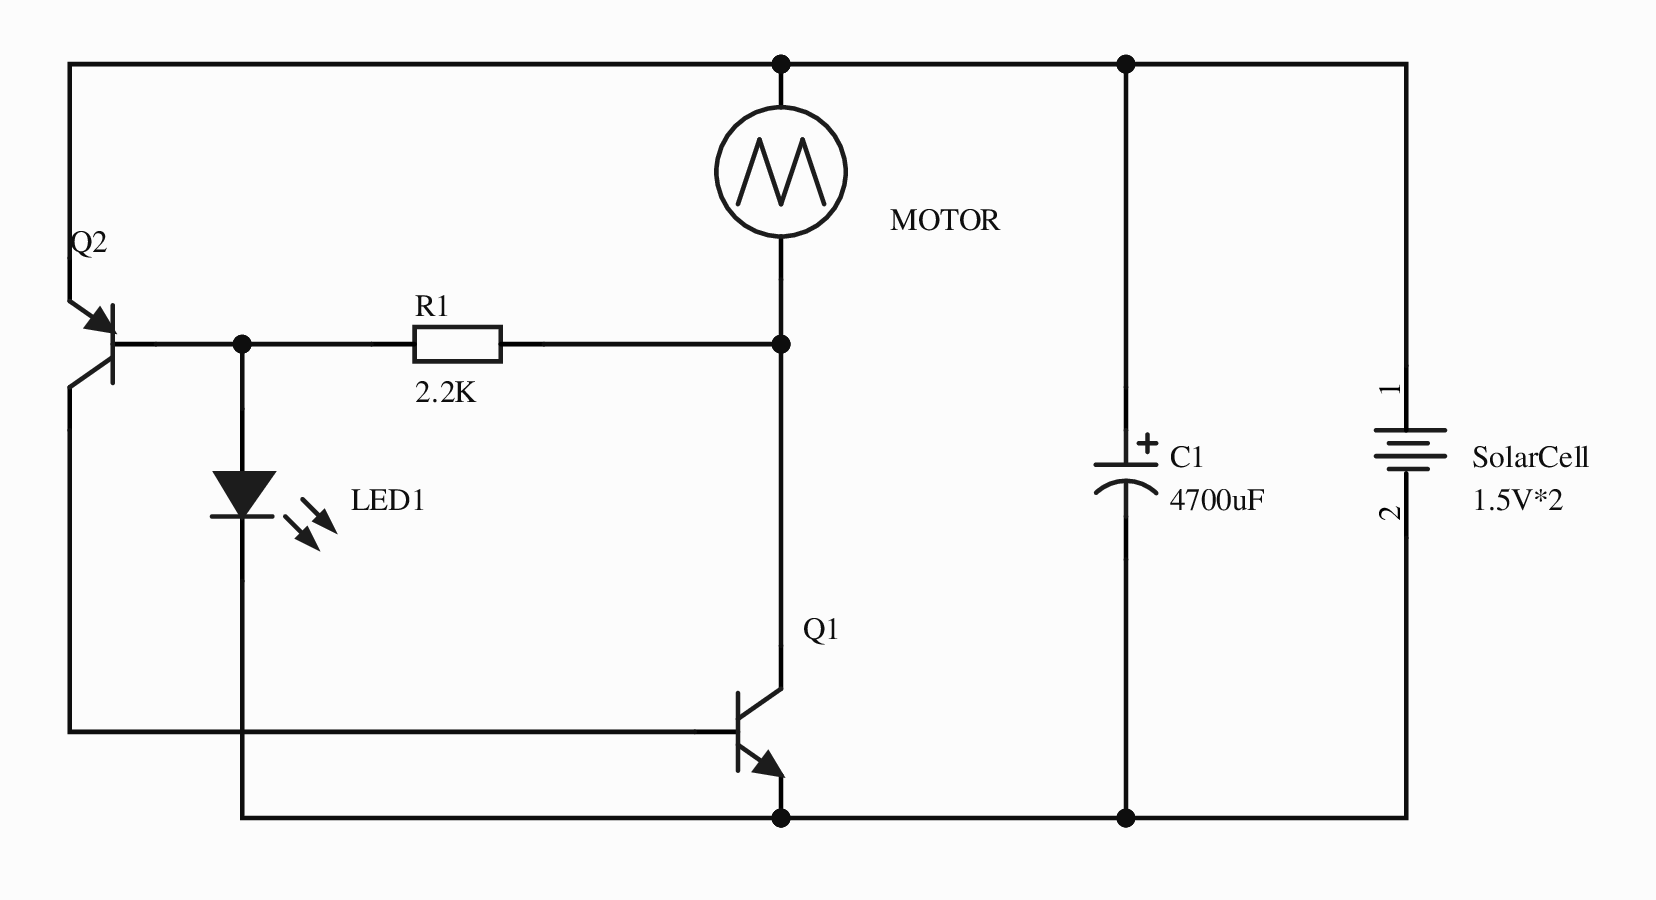
[diagram p0: MISC49939-3.schdoc]
# Altium project MISC49939-2.PrjPcb
1 sheet, 7 parts. Net scope: global (net labels, ports and power ports of the same name join across sheets).
Board file: MISC49939.pcbdoc

## Sheet MISC49939-3.schdoc
size 297 x 209 mm; Version: V1.0; @Project Name: MISC49939; @Update Date: 2026-10-05; @Create Date: 2026-10-05; @Board Name: MISC49939; @Create Time: 20:24:00; @Page Count: 1; @Page No: 1; @Schematic Name: MISC49939; @Update Time: 20:24:00; Size: A4

### Parts
C1  4700uF  [CAP-TH_BD5.0-P2.00-D0.8-FD-10UF50VC110GL]
LED1  (no value)  [LED_0603]
MOTOR  MOTOR_3  [VIBRATING-MOTOR-SMD_3P_C9900012555]  (value not drawn)
Q1  (no value)  [S8050_SOT-23]
Q2  (no value)  [S8550P_SOT]
R1  2.2K  [R0603]
SolarCell  1.5V*2  [BAT-TH_CR2032-2-1]

### Nets
NetC1_1: C1.1 MOTOR.1 Q2.2(E) SolarCell.1
NetC1_2: C1.2 LED1.1(C) Q1.2 SolarCell.2
NetLED1_2: LED1.2(A) Q2.1(B) R1.1
NetMOTOR_2: MOTOR.2 Q1.3 R1.2
NetQ1_1: Q1.1 Q2.3(C)

### Library data of the parts
C1 = 10UF50VC110GL: Capacitance:10uF;Tolerance:±20%;Rated voltage:50V;Ripple current:120mA@100KHz;Equivalent series resistance(ESR):1.6Ω;; Manufacturer: Econd(米朗电子); AddInBom: yes; ModelId: b35ab6b0460c4c43a629d91cfc2b58780819f05c4eef4c71ace90d822a990e87; ModelTransform: 196.85,196.85,0,0,0,0,0,0,-196.85; Tolerance: ±20%; Voltage Rating: 50V; Equivalent Series Resistance(ESR): 1.6Ω; Pin Spacing: 2mm; Lifetime: 5000hrs@105℃; Symbol: 10UF50VC110GL; Device: 10UF50VC110GL; Value: 4700uF; FootprintName: CAP-TH_BD5.0-P2.00-D0.8-FD-10UF50VC110GL; LCSC Part Name: 10uF ±20% 50V; ManufacturerPart: 10UF50VC110GL; Supplier Footprint: 插件,D5xL11mm; JLCPCB Part Class: Extended Part; Datasheet: example.com/datasheet/10UF50VC110GL/49031974.html; Supplier: LCSC; ConvertToPcb: yes; ModelName: CAP-TH_BD5.0-P2.00-D0.8-FD-10UF50VC110GL; Ripple Current: 120mA@100KHz; Diameter: 5mm; Height - Seated (Max): 11mm; Operating Temperature: -40℃~+105℃
LED1 = LED_0603-B: Symbol: LED_B; Convert to PCB: yes; 3D Model: eb8d964598f24248affda46f619856c50819f05c4eef4c71ace90d822a990e87; 3D Model Transform: 63.1,31.6,23.7,0,0,0,0,0,0; ModelName: LED-0603_B; Device: LED_0603-B; Add into BOM: yes; Supplier Footprint: 0603; FootprintName: LED_0603
MOTOR = MOTOR_3: AddInBom: yes; Symbol: MOTOR_3; Device: MOTOR_3; FootprintName: VIBRATING-MOTOR-SMD_3P_C9900012555; LCSC Part Name: MOTOR_3; SupplierPart: C9900022375; ManufacturerPart: MOTOR_3; Supplier Footprint: SHOCK_0408; JLCPCB Part Class: Extended Part; Supplier: LCSC; ConvertToPcb: yes
Q1 = S8050_SOT_NPN: Symbol: NPN; ConvertToPcb: yes; ModelId: c62791f0466c4ae2a892c056b845b0ca0819f05c4eef4c71ace90d822a990e87; ModelName: SOT-23-3P_L2.9-W1.3-H1.0-LS2.4-P0.95; ModelTransform: 98.6,114.12,41.29,180,0,0,0,0,-3; Device: S8050_SOT_NPN; FootprintName: S8050_SOT-23; AddInBom: yes; Supplier Footprint: SOT-23
Q2 = S8550_SOT_PNP: Symbol: PNP; ConvertToPcb: yes; ModelId: 9c0df02d6f3e44e889da37f3e5bf54960819f05c4eef4c71ace90d822a990e87; ModelName: SOT-23-3_L2.9-W1.4-P1.90-LS2.5-BR; ModelTransform: 98.43,114.17,37.91,0,0,0,0,0,0; Device: S8550_SOT_PNP; FootprintName: S8550P_SOT; AddInBom: yes; Supplier Footprint: SOT-23
R1 = Res_0603: Symbol: Resistor; ConvertToPcb: yes; ModelId: fc143cca1e79419f9cd78b61e9279f080819f05c4eef4c71ace90d822a990e87; ModelTransform: 31.8897,63.7794,0,90,0,0,0,0,0; Device: Res_0603; Value: 2.2K; FootprintName: R0603; AddInBom: yes; Supplier Footprint: 0603; ModelName: R0603
SolarCell = CR2032-2-1: AddInBom: yes; ModelId: 9f297eb2328241df835384c32afd7d320819f05c4eef4c71ace90d822a990e87; ModelTransform: 964.565,870.04,0,0,0,0,-42.047,0,-137.795; Symbol: CR2032-2-1; Device: CR2032-2-1; Manufacturer Part: 1.5V*2; FootprintName: BAT-TH_CR2032-2-1; LCSC Part Name: CR2032-2-1; SupplierPart: C9900018737; Supplier Footprint: BATTERY_CR2032-A; JLCPCB Part Class: Extended Part; Supplier: LCSC; ConvertToPcb: yes; ModelName: BAT-TH_CR2032-2-1